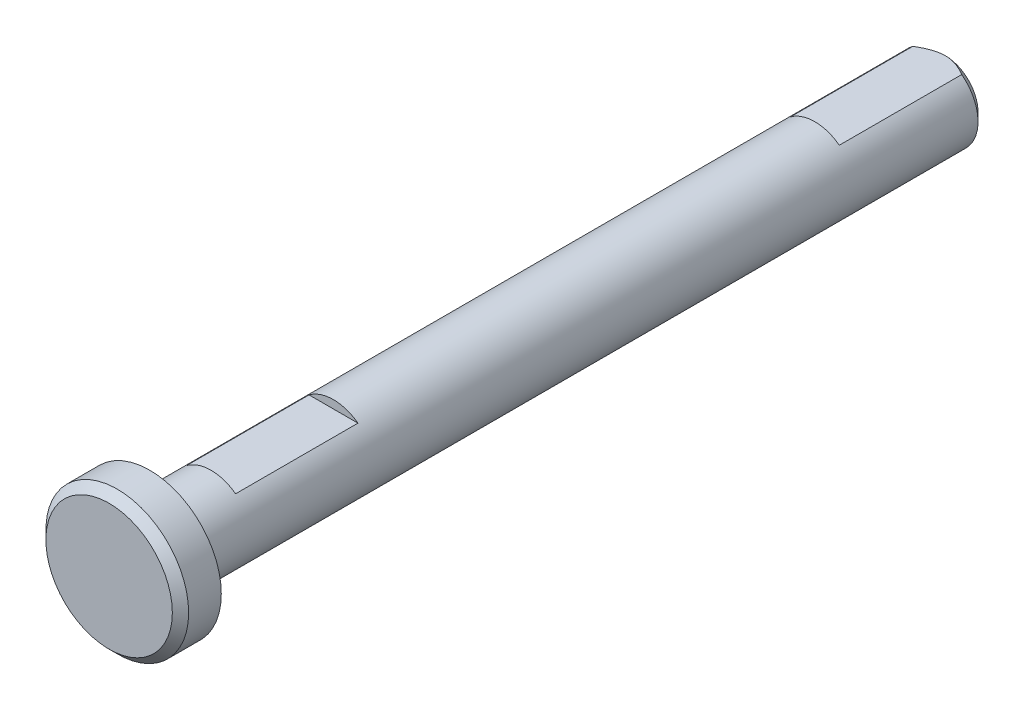
SolidWorks part; units mm, degrees
ref_plane "Front Plane" through (0, 0, 0) normal (0, 0, 1) x (1, 0, 0)
ref_plane "Top Plane" through (0, 0, 0) normal (0, 1, 0) x (1, 0, 0)
ref_plane "Right Plane" through (0, 0, 0) normal (1, 0, 0) x (0, 0, -1)
sketch "Sketch1" plane through (0, 0, 0) normal (0, 0, 1) x (1, 0, 0)
  circle A0 centre (0, 0) radius 1
  dimension "D1" = 2
extrude "Boss-Extrude1" add sketch "Sketch1" along normal mid plane 19.5
sketch "Sketch2" plane through (0, 0, 9.75) normal (0, 0, 1) x (1, 0, 0)
  circle A0 centre (0, 0) radius 1.75
  dimension "D1" = 3.5
extrude "Boss-Extrude2" add sketch "Sketch2" along normal blind 1
chamfer "Chamfer1" distance 0.2 angle 45 2 edges at (1, 0, -9.75) (1.75, 0, 10.75)
sketch "Sketch3" plane through (0, 0, -9.75) normal (0, 0, -1) x (-1, 0, 0)
  line L0 (-0.6, 0.8) -> (0.6, 0.8)
  circle A0 centre (0, 0) radius 1 construction
  arc A1 (0.6, 0.8) -> (-0.6, 0.8) centre (0, 0) ccw
  dimension "D1" = 0.8
extrude "Cut-Extrude1" cut sketch "Sketch3" against normal blind 3.2
ref_plane "Plane1" through (0, 0, 6.75) normal (0, 0, -1) x (-1, 0, 0)
sketch "Sketch4" plane through (0, 0, 6.75) normal (0, 0, -1) x (-1, 0, 0)
  line L0 (-0.6, 0.8) -> (0.6, 0.8) construction
  line L1 (-0.6, 0.8) -> (0.6, 0.8)
  circle A0 centre (0, 0) radius 1 construction
  arc A1 (0.6, 0.8) -> (-0.6, 0.8) centre (0, 0) ccw
extrude "Cut-Extrude2" cut sketch "Sketch4" against normal mid plane 3
